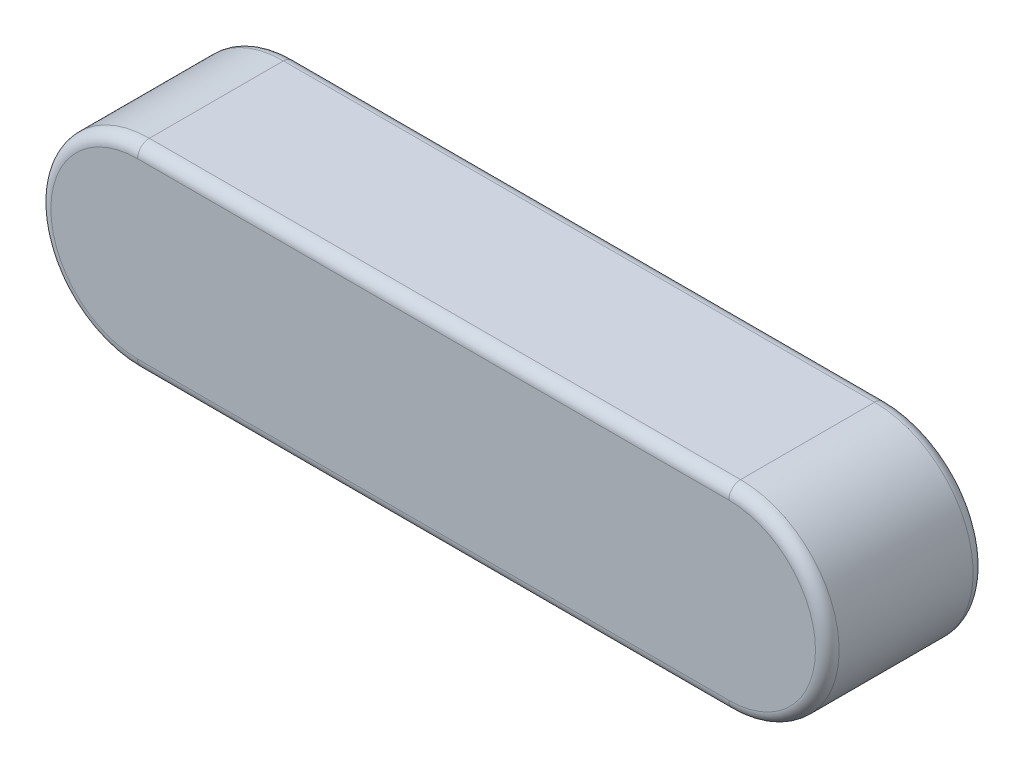
from build123d import *

# Parameters (mm, degrees)
EXTRUDE_523_DEPTH = 8
FILLET_1_R        = 0.6


with BuildPart() as part:
    # 草图1 → Extrude 523 (new body)
    with BuildSketch(Plane.XY):
        with BuildLine():
            Line((-15, 5), (15, 5))
            ThreePointArc((15, 5), (20, 0), (15, -5))
            Line((15, -5), (-15, -5))
            ThreePointArc((-15, -5), (-20, 0), (-15, 5))
        make_face()
    extrude(amount=EXTRUDE_523_DEPTH)

    # 圆角1
    fillet_1_edges = [part.edges().sort_by_distance(p)[0] for p in [
        (20, 0, 8),
        (0, 5, 8),
        (-20, 0, 8),
        (0, 5, 0),
        (20, 0, 0),
        (0, -5, 0),
        (-20, 0, 0),
        (0, -5, 8),
    ]]
    fillet(fillet_1_edges, radius=FILLET_1_R)


solid = part.part
